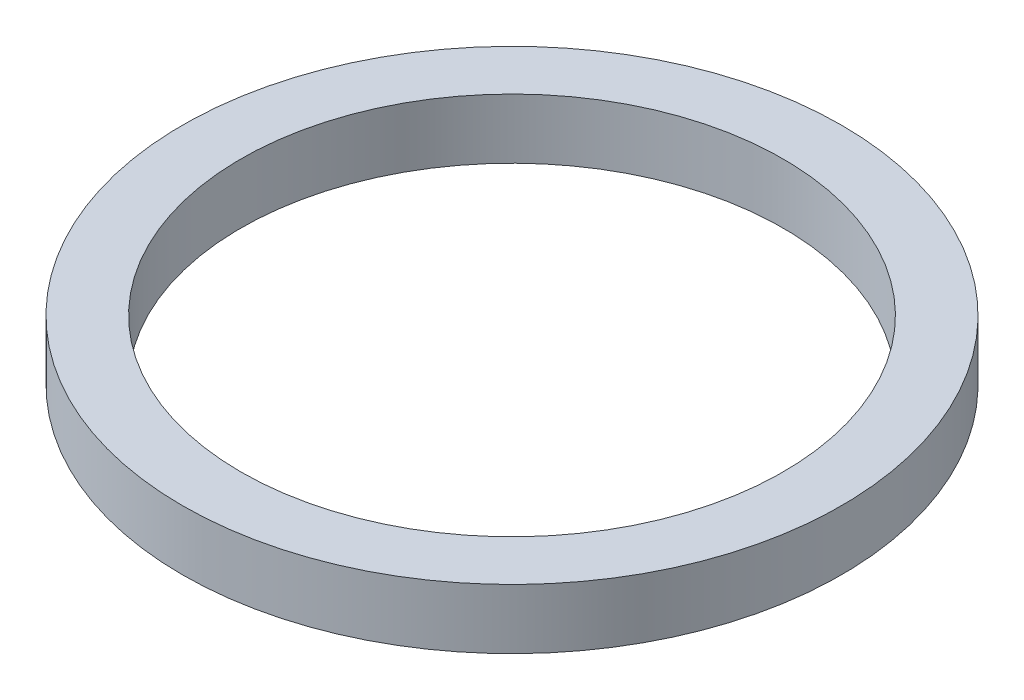
SolidWorks part; units mm, degrees
material "哈碳纤"
ref_plane "前视基准面" through (0, 0, 0) normal (0, 0, 1) x (1, 0, 0)
ref_plane "上视基准面" through (0, 0, 0) normal (0, 1, 0) x (1, 0, 0)
ref_plane "右视基准面" through (0, 0, 0) normal (1, 0, 0) x (0, 0, -1)
other "Configuration Table"
sketch "草图1" plane through (0, 0, 0) normal (0, 1, 0) x (1, 0, 0)
  circle A0 centre (0, 0) radius 13.575
  circle A1 centre (0, 0) radius 16.5
  dimension "D1" = 27.15
  dimension "D2" = 33
extrude "凸台-拉伸1" add sketch "草图1" along normal blind 3
